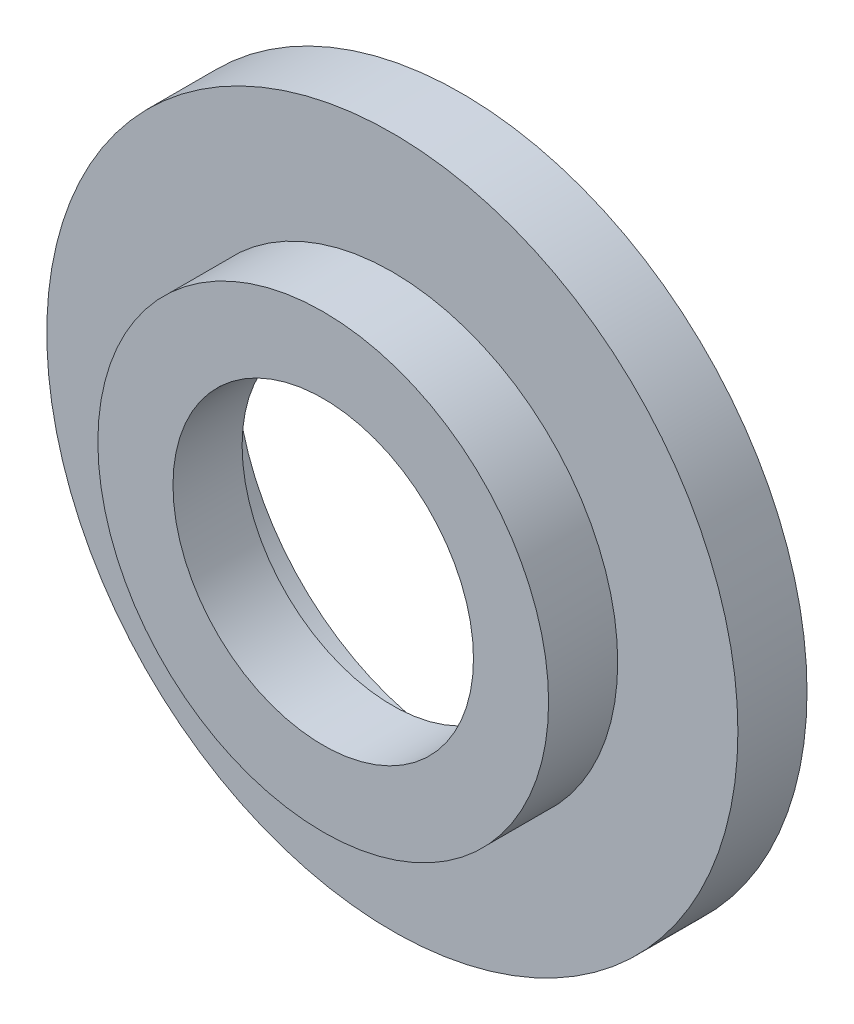
from build123d import *

# Parameters (mm, degrees)
SKETCH_1_R      = 11.5
SKETCH_1_R_2    = 7.5
EXTRUDE_1_DEPTH = 2.3
SKETCH_2_R      = 7.5
SKETCH_2_R_2    = 5
EXTRUDE_2_DEPTH = 2.3


with BuildPart() as part:
    # 草图1 → 凸台-拉伸1 (new body)
    with BuildSketch(Plane.XY):
        Circle(SKETCH_1_R)
        Circle(SKETCH_1_R_2, mode=Mode.SUBTRACT)
    extrude(amount=EXTRUDE_1_DEPTH)


with BuildPart() as body_2:
    # 草图2 → 凸台-拉伸2 (new body)
    with BuildSketch(Plane.XY.offset(2.3)):
        Circle(SKETCH_2_R)
        Circle(SKETCH_2_R_2, mode=Mode.SUBTRACT)
    extrude(amount=EXTRUDE_2_DEPTH)


solid = Compound([part.part, body_2.part])
